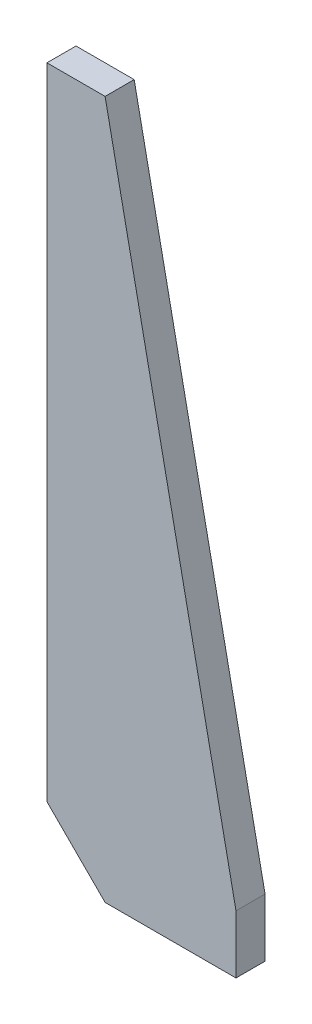
SolidWorks part; units mm, degrees
material "Q235B"
ref_plane "Front Plane" through (0, 0, 0) normal (0, 0, 1) x (1, 0, 0)
ref_plane "Top Plane" through (0, 0, 0) normal (0, 1, 0) x (1, 0, 0)
ref_plane "Right Plane" through (0, 0, 0) normal (1, 0, 0) x (0, 0, -1)
sketch "Sketch1" plane through (0, 0, 0) normal (0, 0, 1) x (1, 0, 0)
  line L0 (0, 0) -> (65, 0)
  line L1 (65, 0) -> (65, 20)
  line L2 (65, 20) -> (20, 240)
  line L3 (20, 240) -> (0, 240)
  line L4 (0, 240) -> (0, 0)
  dimension "D1" = 65
  dimension "D2" = 20
  dimension "D3" = 20
  dimension "D4" = 240
extrude "Boss-Extrude1" add sketch "Sketch1" along normal mid plane 10
chamfer "Chamfer1" distance 20 angle 45 1 edges at (0, 0, 0)
